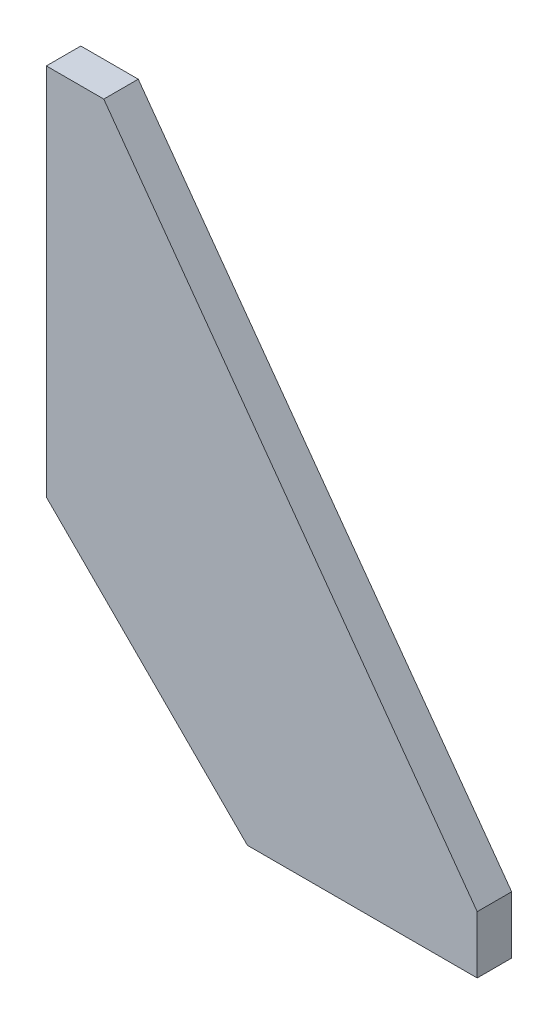
from build123d import *

# Parameters (mm, degrees)
BOSS_EXTRUDE1_DEPTH = 3
CHAMFER1_SIZE       = 35


with BuildPart() as part:
    # Sketch1 → Boss-Extrude1 (new, symmetric)
    with BuildSketch(Plane.XY):
        Polygon((0, 100), (0, 0), (75, 0), (75, 10), (10, 100), align=None)
    extrude(amount=BOSS_EXTRUDE1_DEPTH, both=True)

    # Chamfer1
    chamfer1_edges = [part.edges().sort_by_distance(p)[0] for p in [
        (0, 0, 0),
    ]]
    chamfer(chamfer1_edges, length=CHAMFER1_SIZE)


solid = part.part
